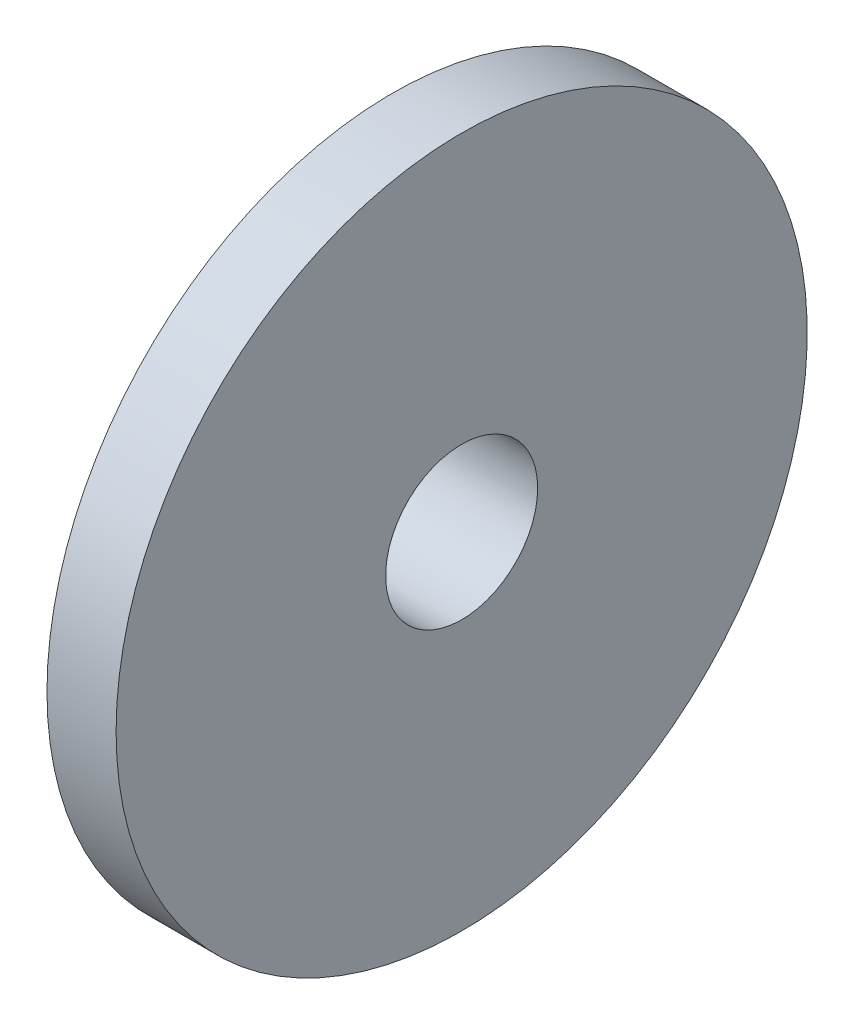
from build123d import *

# Parameters (mm, degrees)
SKETCH2_R          = 5.5
CUT_EXTRUDE1_DEPTH = 17


with BuildPart() as part:
    # Sketch1 → Revolve1 (revolve)
    with BuildSketch(Plane.XY, mode=Mode.PRIVATE) as revolve1_sk:
        Polygon((0, 0), (0, 15), (7, 15), (7, 25), (12, 25), (12, 0), align=None)
    revolve(revolve1_sk.sketch.rotate(Axis((0, 0, 0), (1, 0, 0)), 90), axis=Axis((0, 0, 0), (1, 0, 0)))

    # Sketch2 → Cut-Extrude1 (cut)
    with BuildSketch(Plane(origin=(12, 0, 0), x_dir=(0, 0, -1), z_dir=(1, 0, 0))):
        Circle(SKETCH2_R)
    extrude(amount=-CUT_EXTRUDE1_DEPTH, mode=Mode.SUBTRACT)


solid = part.part
